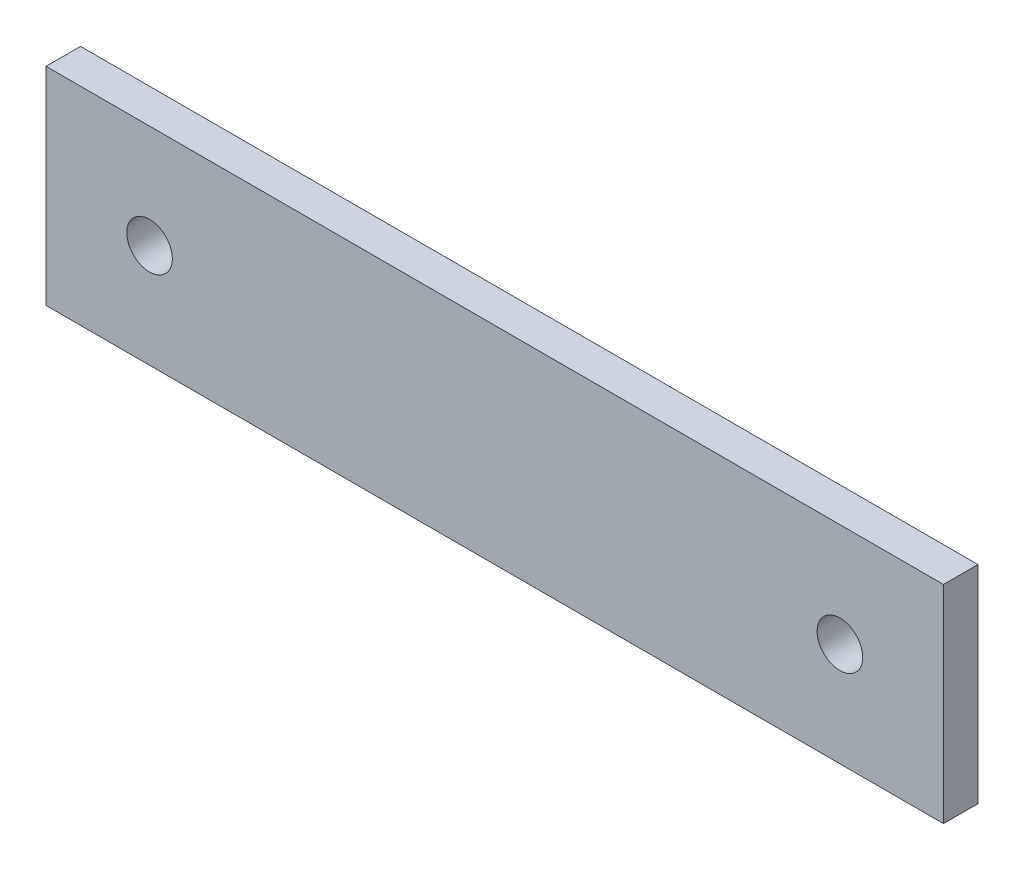
SolidWorks part; units mm, degrees
ref_plane "前视基准面" through (0, 0, 0) normal (0, 0, 1) x (1, 0, 0)
ref_plane "上视基准面" through (0, 0, 0) normal (0, 1, 0) x (1, 0, 0)
ref_plane "右视基准面" through (0, 0, 0) normal (1, 0, 0) x (0, 0, -1)
sketch "草图1" plane through (0, 0, 0) normal (0, 0, 1) x (1, 0, 0)
  line L0 (-50, 0) -> (0, 0) construction
  line L1 (65, -15) -> (-65, -15)
  line L2 (65, -15) -> (65, 15)
  line L3 (65, 15) -> (-65, 15)
  line L4 (-65, -15) -> (-65, 15)
  line L5 (65, -15) -> (-65, 15) construction
  line L6 (65, 15) -> (-65, -15) construction
  line L7 (0, 0) -> (50, 0) construction
  circle A0 centre (-50, 0) radius 3.3
  circle A1 centre (50, 0) radius 3.3
  point P0 (0, 0)
  dimension "D3" = 6.6
  dimension "D1" = 130
  dimension "D2" = 30
  dimension "D4" = 50
extrude "凸台-拉伸1" add sketch "草图1" along normal blind 5
